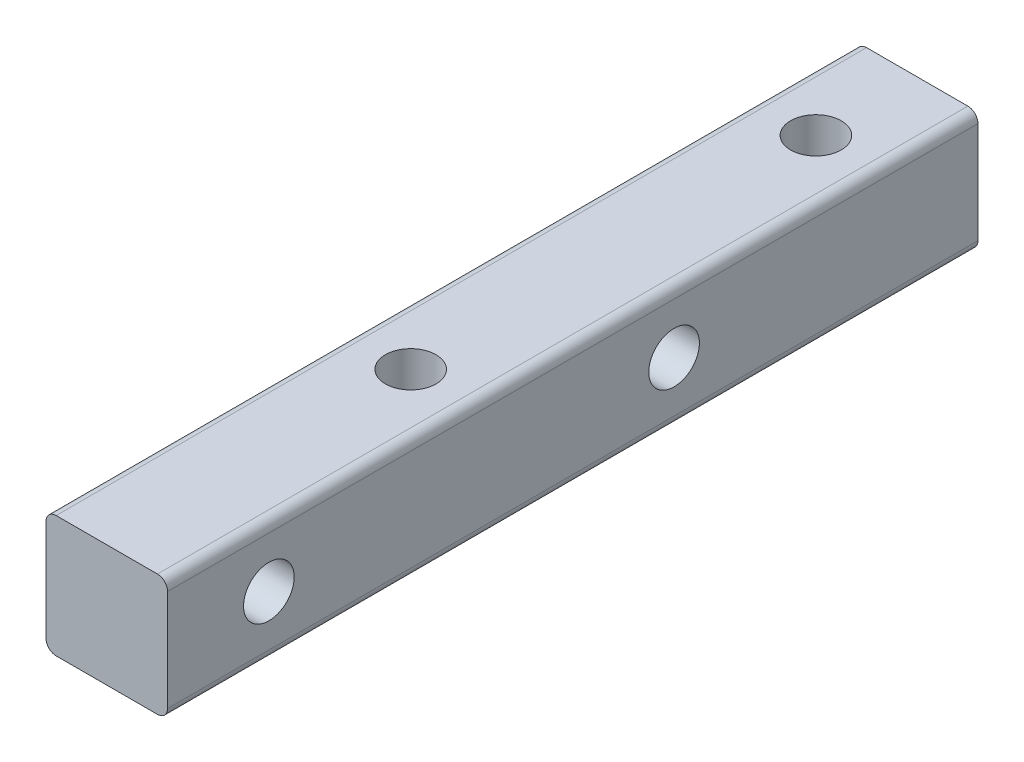
SolidWorks part; units mm, degrees
material "6061 合金"
ref_plane "前视基准面" through (0, 0, 0) normal (0, 0, 1) x (1, 0, 0)
ref_plane "上视基准面" through (0, 0, 0) normal (0, 1, 0) x (1, 0, 0)
ref_plane "右视基准面" through (0, 0, 0) normal (1, 0, 0) x (0, 0, -1)
sketch "草图1" plane through (0, 0, 0) normal (0, 0, 1) x (1, 0, 0)
  line L1 (-3, -3) -> (3, -3)
  line L2 (-3, -3) -> (-3, 3)
  line L3 (-3, 3) -> (3, 3)
  line L4 (3, -3) -> (3, 3)
  line L5 (-3, -3) -> (3, 3) construction
  line L6 (-3, 3) -> (3, -3) construction
  point P0 (0, 0)
  dimension "D1" = 6
extrude "凸台-拉伸1" add sketch "草图1" along normal mid plane 40
sketch "草图2" plane through (0, 3, 0) normal (0, 1, 0) x (1, 0, 0)
  line L0 (0, -20) -> (0, 20) construction
  line L1 (3, -20) -> (-3, -20) construction
  line L2 (3, 20) -> (-3, 20) construction
  point P6 (0, 15)
  point P7 (0, -5)
  dimension "D1" = 5
  dimension "D2" = 20
hole_wizard "M3 螺纹孔1" positions "草图3" profile "草图4" tap size "M3" standard "GB" end condition through all
sketch "草图3" plane through (0, 3, 0) normal (0, 1, 0) x (1, 0, 0)
  point P0 (0, 15)
  point P3 (0, -5)
sketch "草图4" plane through (0, 3, -15) normal (1, 0, 0) x (0, 0, 1)
  line L0 (0, 0) -> (0, 6)
  line L1 (0, 6) -> (1.25, 6)
  line L2 (1.25, 6) -> (1.25, 0)
  line L5 (1.25, 0) -> (0, 0)
  line L11 (0, -6.35) -> (0, 107.95) construction
  dimension "通孔螺纹孔钻头直径" = 2.5
  dimension "通孔螺纹孔钻头深度" = 6
cosmetic thread "孔螺蚊线1" parameters "D2"=3
cosmetic thread "孔螺蚊线2" parameters "D2"=3
sketch "草图5" plane through (3, 0, 0) normal (1, 0, 0) x (0, 0, -1)
  line L0 (-20, 0) -> (20, 0) construction
  line L1 (-20, -3) -> (-20, 3) construction
  line L2 (20, -3) -> (20, 3) construction
  point P6 (-15, 0)
  point P7 (5, 0)
  dimension "D1" = 5
  dimension "D2" = 20
hole_wizard "M3 螺纹孔2" positions "草图6" profile "草图7" tap size "M3" standard "GB" end condition through all
sketch "草图6" plane through (3, 0, 0) normal (1, 0, 0) x (0, 0, -1)
  point P0 (-15, 0)
  point P3 (5, 0)
sketch "草图7" plane through (3, 0, 15) normal (0, 1, 0) x (0, 0, -1)
  line L0 (0, 0) -> (0, 6)
  line L1 (0, 6) -> (1.25, 6)
  line L2 (1.25, 6) -> (1.25, 0)
  line L5 (1.25, 0) -> (0, 0)
  line L11 (0, -6.35) -> (0, 107.95) construction
  dimension "通孔螺纹孔钻头直径" = 2.5
  dimension "通孔螺纹孔钻头深度" = 6
cosmetic thread "孔螺蚊线3" parameters "D2"=3
cosmetic thread "孔螺蚊线4" parameters "D2"=3
fillet "圆角1" radius 0.5 4 edges at (3, -3, 0) (-3, -3, 0) (-3, 3, 0) (3, 3, 0)
